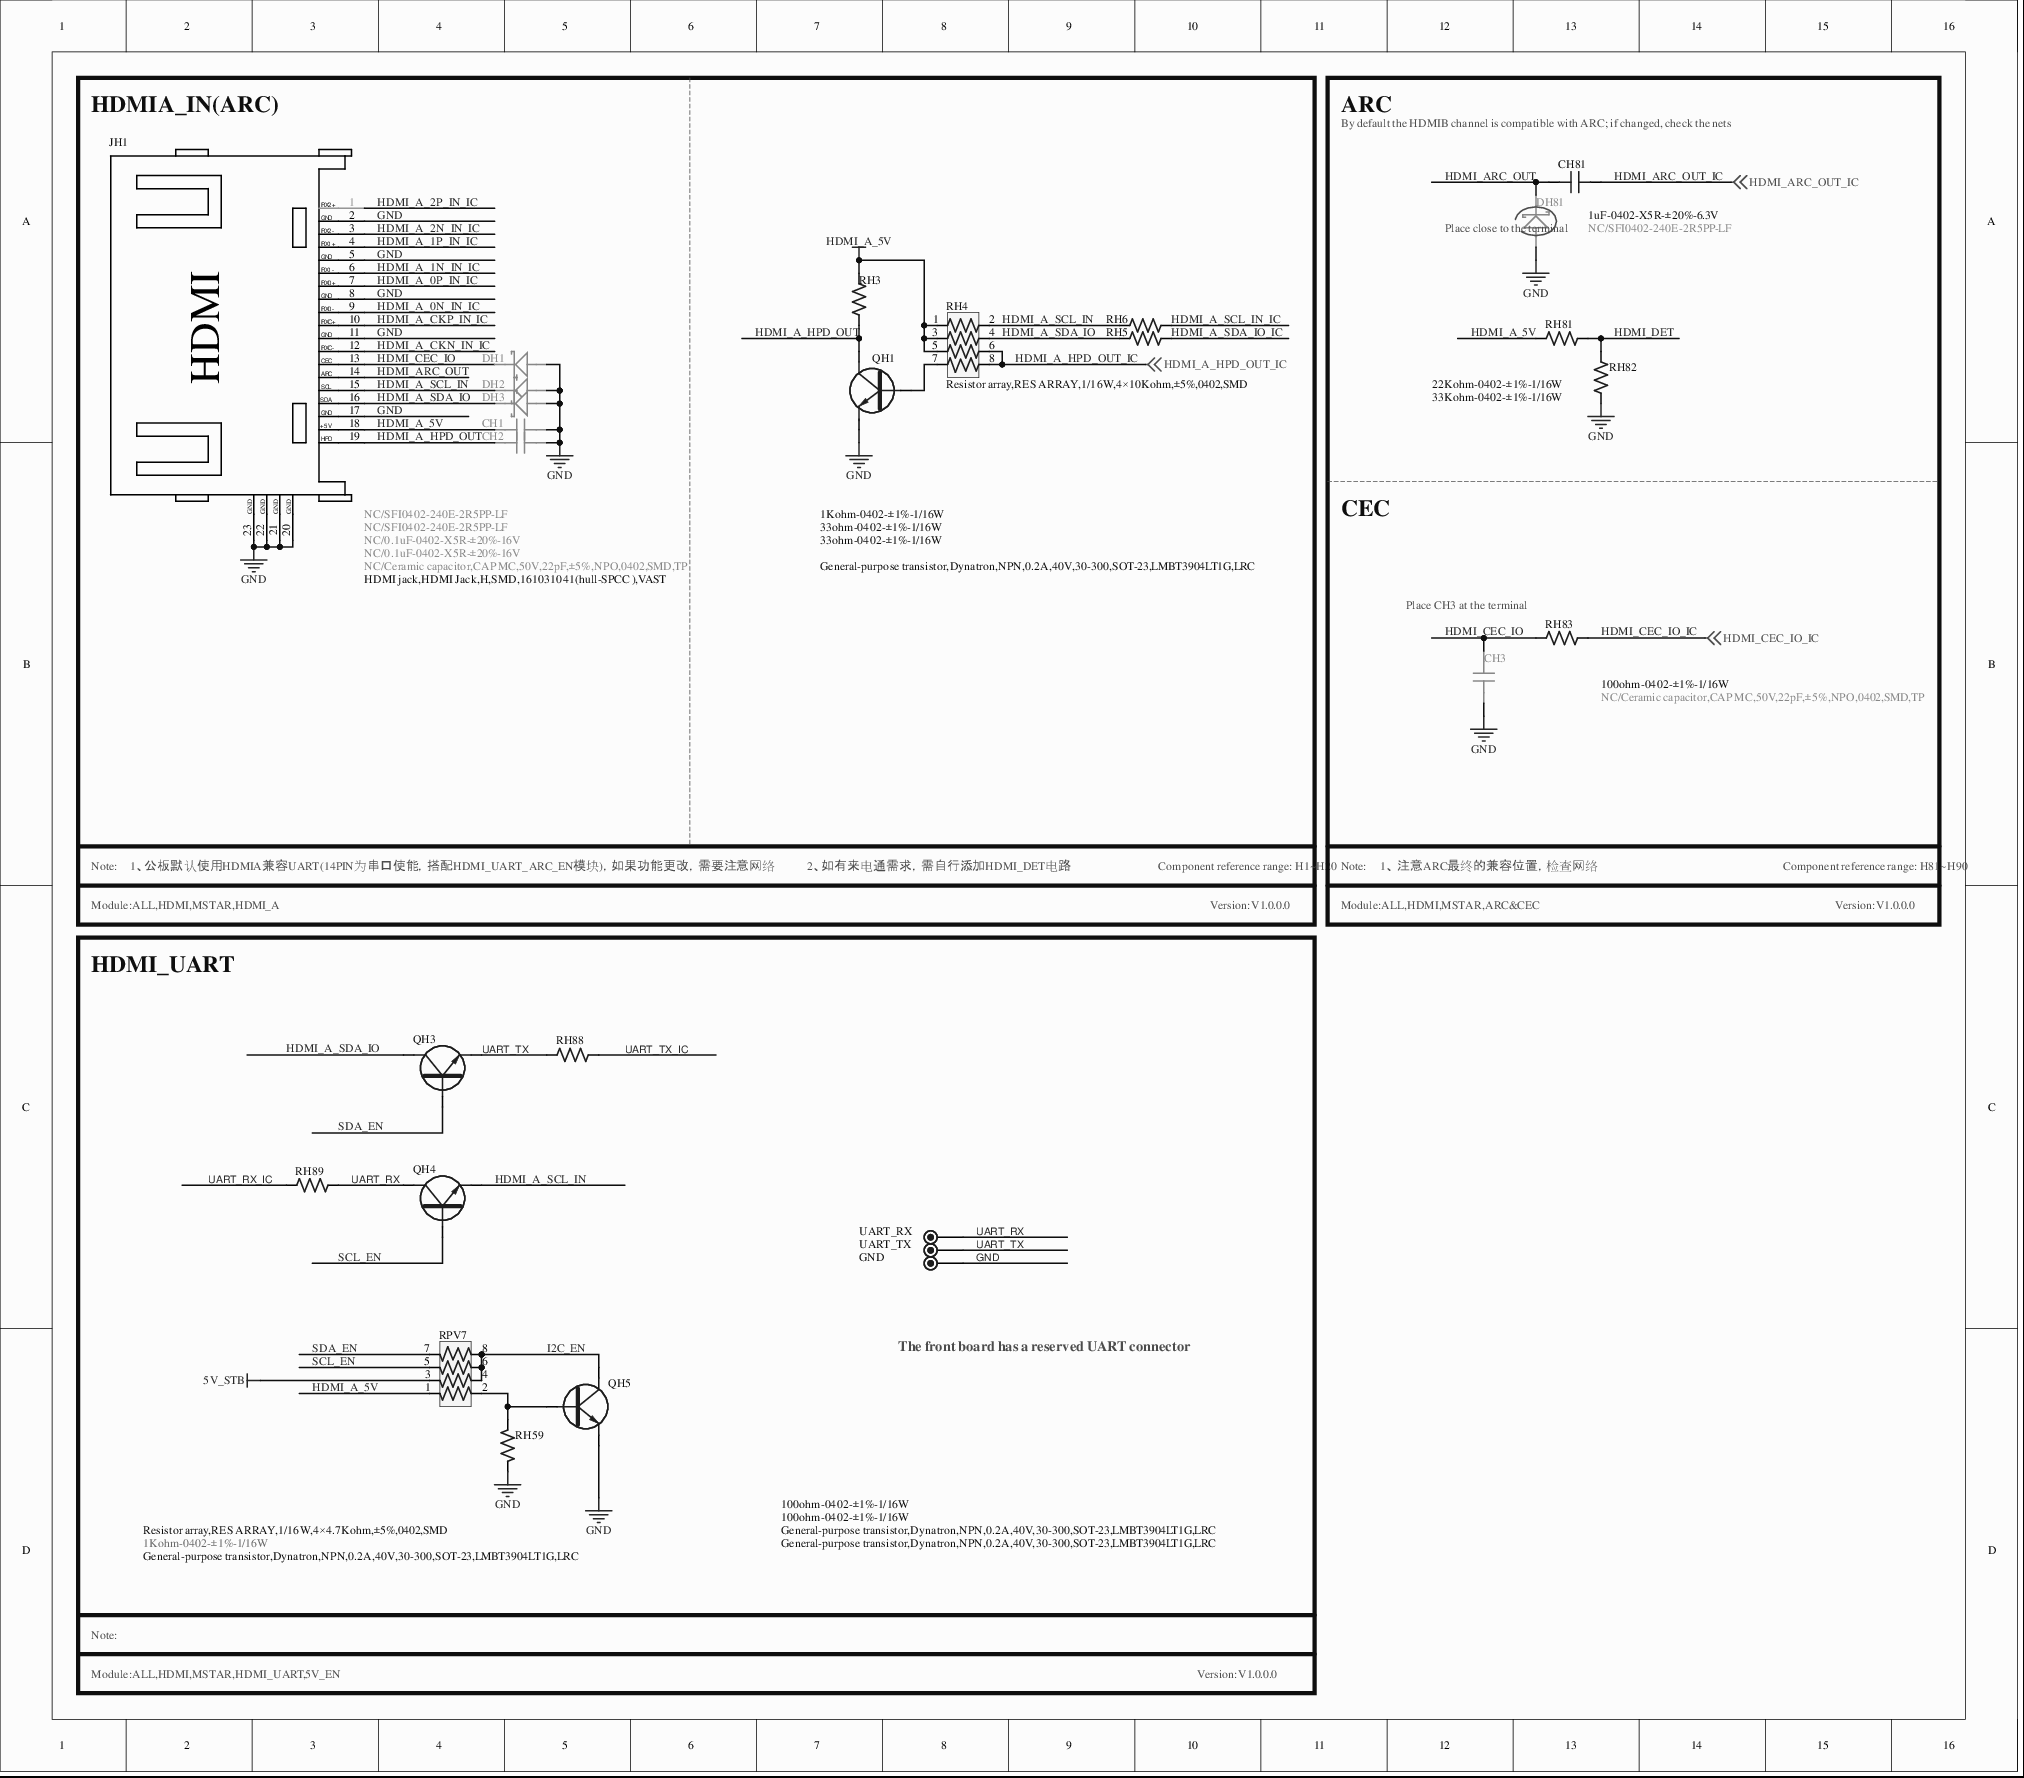
[diagram p0: MISC116569-11.SchDoc]
# Altium project MISC116569-15.PrjPCB (part 6 of 8)

## Sheet MISC116569-11.SchDoc
size 393 x 345 mm

### Parts
CH1  NC/0.1uF-0402-X5R-±20%-16V  [C0402]
CH2  NC/0.1uF-0402-X5R-±20%-16V  [C0402]
CH3  NC/Ceramic capacitor,CAP MC,50V,22pF,±5%,NPO,0402,SMD,TP  [C0402]
CH81  1uF-0402-X5R-±20%-6.3V  [C0402]
DH1  NC/Ceramic capacitor,CAP MC,50V,22pF,±5%,NPO,0402,SMD,TP  [DIODE-S0402]
DH2  NC/SFI0402-240E-2R5PP-LF  [DIODE-S0402]
DH3  NC/SFI0402-240E-2R5PP-LF  [DIODE-S0402]
DH81  NC/SFI0402-240E-2R5PP-LF  [DIODE-S0402]
GND  (no value)  [TP]
JH1  HDMI jack,HDMI Jack,H,SMD,161031041(hull-SPCC ),VAST  [HDMI-HS-1]
QH1  General-purpose transistor,Dynatron,NPN,0.2A,40V,30-300,SOT-23,LMBT3904LT1G,LRC  [SOT-23]
QH3  General-purpose transistor,Dynatron,NPN,0.2A,40V,30-300,SOT-23,LMBT3904LT1G,LRC  [SOT-23]
QH4  General-purpose transistor,Dynatron,NPN,0.2A,40V,30-300,SOT-23,LMBT3904LT1G,LRC  [SOT-23]
QH5  General-purpose transistor,Dynatron,NPN,0.2A,40V,30-300,SOT-23,LMBT3904LT1G,LRC  [SOT-23]
RH3  1Kohm-0402-±1%-1/16W  [R0402]
RH4  Resistor array,RES ARRAY,1/16W,4×10Kohm,±5%,0402,SMD  [RA0402]
RH5  33ohm-0402-±1%-1/16W  [R0402]
RH6  33ohm-0402-±1%-1/16W  [R0402]
RH59  1Kohm-0402-±1%-1/16W  [R0402]
RH81  22Kohm-0402-±1%-1/16W  [R0402]
RH82  33Kohm-0402-±1%-1/16W  [R0402]
RH83  100ohm-0402-±1%-1/16W  [R0402]
RH88  100ohm-0402-±1%-1/16W  [R0402]
RH89  100ohm-0402-±1%-1/16W  [R0402]
RPV7  Resistor array,RES ARRAY,1/16W,4×4.7Kohm,±5%,0402,SMD  [RA0402]
UART_RX  (no value)  [TP]
UART_TX  (no value)  [TP]

### Blocks framed on the sheet
HDMIA_IN(ARC): CH1 CH2 DH1-DH3 JH1 QH1 RH3-RH6
HDMI_UART: GND QH3-QH5 RH59 RH88 RH89 RPV7 UART_RX UART_TX

### Nets
5V_STB: RPV7.3
GND: CH1.2 CH2.2 CH3.1 DH1.A DH2.A DH3.A DH81.A GND.1 JH1.2 JH1.5 JH1.8 JH1.11 JH1.17 JH1.20 JH1.21 JH1.22 JH1.23 QH1.E QH5.E RH59.1 RH82.2
HDMI_A_5V: CH1.1 JH1.18 RH3.2 RH4.1 RH4.3 RH4.5 RH81.2 RPV7.1
HDMI_A_0N_IN_IC: JH1.9
HDMI_A_0P_IN_IC: JH1.7
HDMI_A_1N_IN_IC: JH1.6
HDMI_A_1P_IN_IC: JH1.4
HDMI_A_2N_IN_IC: JH1.3
HDMI_A_2P_IN_IC: JH1.1
HDMI_A_CKN_IN_IC: JH1.12
HDMI_A_CKP_IN_IC: JH1.10
HDMI_A_HPD_OUT: CH2.1 JH1.19 QH1.C RH3.1
HDMI_A_HPD_OUT_IC: RH4.6 RH4.8 ; off-sheet HDMI_A_HPD_OUT_IC
HDMI_A_SCL_IN: DH2.K JH1.15 QH4.E RH4.2 RH6.1
HDMI_A_SCL_IN_IC: RH6.2
HDMI_A_SDA_IO: DH3.K JH1.16 QH3.C RH4.4 RH5.1
HDMI_A_SDA_IO_IC: RH5.2
HDMI_ARC_OUT: CH81.1 DH81.K JH1.14
HDMI_ARC_OUT_IC: CH81.2 ; off-sheet HDMI_ARC_OUT_IC
HDMI_CEC_IO: CH3.2 DH1.K JH1.13 RH83.2
HDMI_CEC_IO_IC: RH83.1 ; off-sheet HDMI_CEC_IO_IC
HDMI_DET: RH81.1 RH82.1
I2C_EN: QH5.C RPV7.4 RPV7.6 RPV7.8
SCL_EN: QH4.B RPV7.5
SDA_EN: QH3.B RPV7.7
UART_RX: QH4.C RH89.1 UART_RX.1
UART_RX_IC: RH89.2
UART_TX: QH3.E RH88.2 UART_TX.1
UART_TX_IC: RH88.1
NetQH1_B: QH1.B RH4.7
NetQH5_B: QH5.B RH59.2 RPV7.2

### Notes on the sheet
- ARC
- By default the HDMIB channel is compatible with ARC; if changed, check the nets
- (near DH81) Place close to the terminal
- CEC
- (near RH83) Place CH3 at the terminal
- Note:
- 1、公板默认使用HDMIA兼容UART(14PIN为串口使能，搭配HDMI_UART_ARC_EN模块)，如果功能更改，需要注意网络
- 2、如有来电通需求，需自行添加HDMI_DET电路
- Component reference range: H1~H20
- 1、 注意ARC最终的兼容位置，检查网络
- Component reference range: H81~H90
- Module:ALL,HDMI,MSTAR,HDMI_A
- Version:V1.0.0.0
- Module:ALL,HDMI,MSTAR,ARC&CEC
- The front board has a reserved UART connector
- Module:ALL,HDMI,MSTAR,HDMI_UART,5V_EN

### Library data of the parts
CH1 CH2 = 0.1uF-0402-X5R-±20%-16V-D
CH3 = 004.003.0000530-D: Ceramic capacitor,CAP MC,50V,22pF,±5%,NPO,0402,SMD,TP-D
CH81 = 1uF-0402-X5R-±20%-6.3V-D
DH1-DH3 DH81 = 004.005.0000315-D: TVS diode,DIO ESD,2.5pF,200V,0402,SMD,SFI0402-240E-2R5PP-LF,SFI-D
GND UART_RX UART_TX = TEST
JH1 = XXX.XXX.0001122-D: HDMI jack,HDMI Jack,H,SMD,161031041(hull-SPCC ),VAST-D
QH1 = 004.006.0000007-D: General-purpose transistor,Dynatron,NPN,0.2A,40V,60-300,SOT-23,KMBT3904,KEXIN-D
QH3-QH5 = LMBT3904LT1G-D-NPN: Q-NPN-#-#-#
RH3 = 1Kohm-0402-±5%-1/16W-D
RH4 RPV7 = 4*100ohm-0402-±5%-1/16W-D
RH5 RH6 = 33ohm-0402-±5%-1/16W-D
RH59 = 10Kohm-0402-±5%-1/16W-D
RH81 = 22Kohm-0402-±5%-1/16W-D
RH82 = 33Kohm-0402-±5%-1/16W-D
RH83 RH88 RH89 = 004.002.0000568-D: Thick-film resistor,RES,1/16W,100ohm,±5%,0402,SMD-D

## Sheet MISC116569-12.SchDoc
size 294 x 215 mm
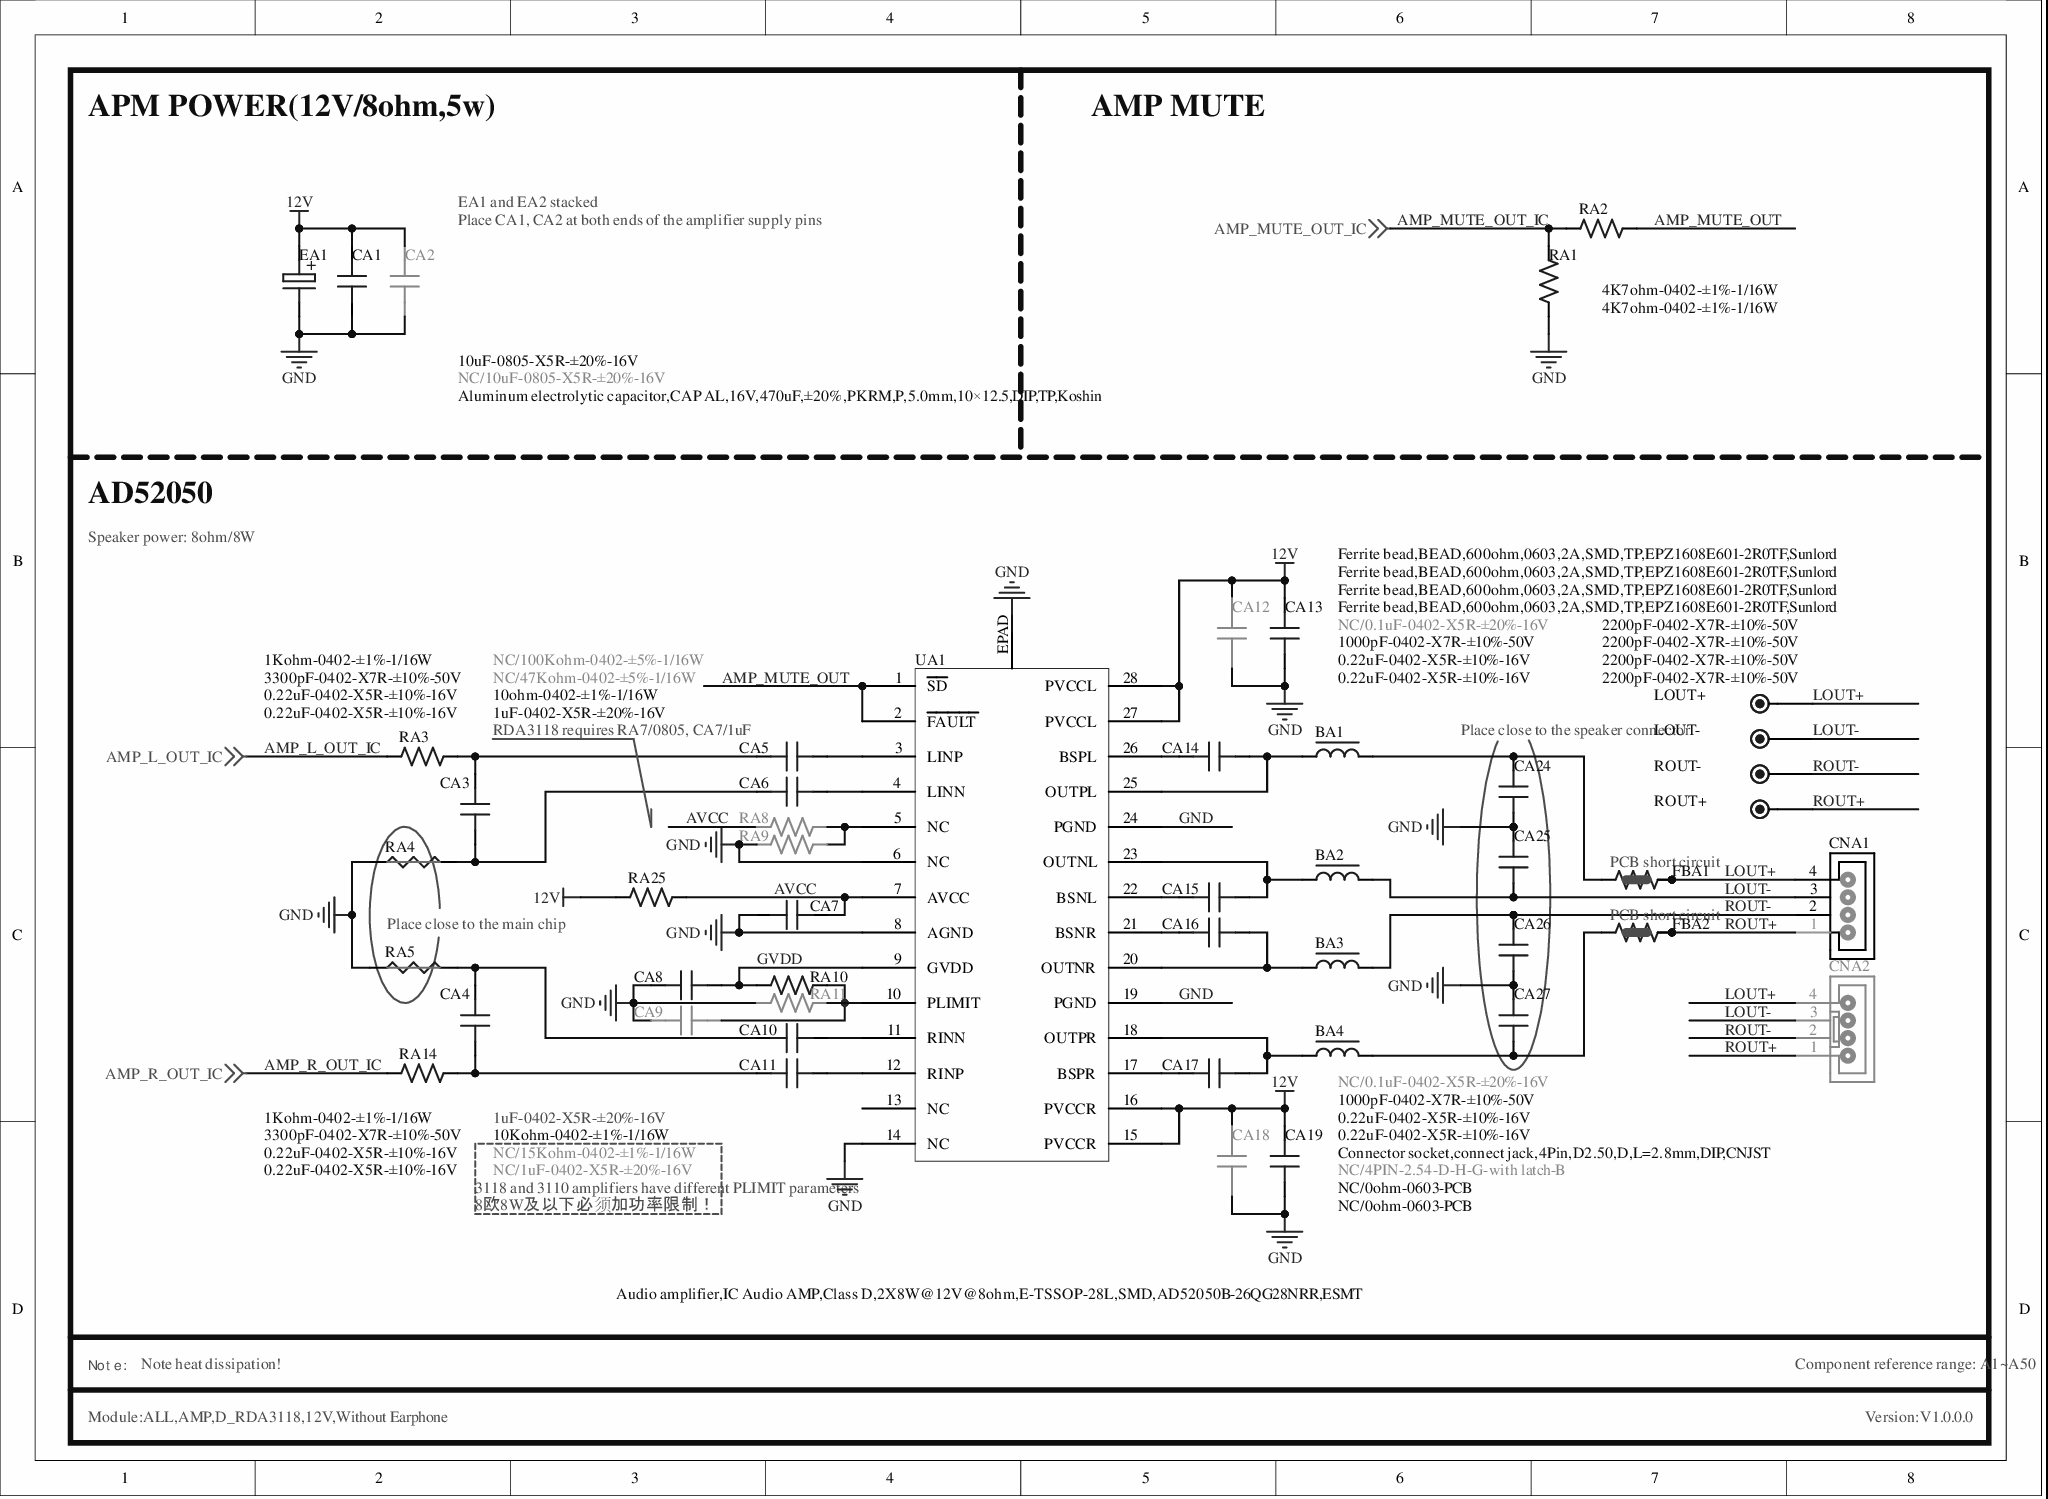
[diagram p1: MISC116569-12.SchDoc]

### Parts
BA1  Ferrite bead,BEAD,600ohm,0603,2A,SMD,TP,EPZ1608E601-2R0TF,Sunlord  [L0603]
BA2  Ferrite bead,BEAD,600ohm,0603,2A,SMD,TP,EPZ1608E601-2R0TF,Sunlord  [L0603]
BA3  Ferrite bead,BEAD,600ohm,0603,2A,SMD,TP,EPZ1608E601-2R0TF,Sunlord  [L0603]
BA4  Ferrite bead,BEAD,600ohm,0603,2A,SMD,TP,EPZ1608E601-2R0TF,Sunlord  [L0603]
CA1  10uF-0805-X5R-±20%-16V  [C0805]
CA2  NC/10uF-0805-X5R-±20%-16V  [C0805]
CA3  3300pF-0402-X7R-±10%-50V  [C0402]
CA4  3300pF-0402-X7R-±10%-50V  [C0402]
CA5  0.22uF-0402-X5R-±10%-16V  [C0402]
CA6  0.22uF-0402-X5R-±10%-16V  [C0402]
CA7  1uF-0402-X5R-±20%-16V  [C0402]
CA8  1uF-0402-X5R-±20%-16V  [C0402]
CA9  NC/1uF-0402-X5R-±20%-16V  [C0402]
CA10  0.22uF-0402-X5R-±10%-16V  [C0402]
CA11  0.22uF-0402-X5R-±10%-16V  [C0402]
CA12  NC/0.1uF-0402-X5R-±20%-16V  [C0402]
CA13  1000pF-0402-X7R-±10%-50V  [C0402]
CA14  0.22uF-0402-X5R-±10%-16V  [C0402]
CA15  0.22uF-0402-X5R-±10%-16V  [C0402]
CA16  0.22uF-0402-X5R-±10%-16V  [C0402]
CA17  0.22uF-0402-X5R-±10%-16V  [C0402]
CA18  NC/0.1uF-0402-X5R-±20%-16V  [C0402]
CA19  1000pF-0402-X7R-±10%-50V  [C0402]
CA24  2200pF-0402-X7R-±10%-50V  [C0402]
CA25  2200pF-0402-X7R-±10%-50V  [C0402]
CA26  2200pF-0402-X7R-±10%-50V  [C0402]
CA27  2200pF-0402-X7R-±10%-50V  [C0402]
CNA1  Connector socket,connect jack,4Pin,D2.50,D,L=2.8mm,DIP,CNJST  [SIP4/2.54D-1]
CNA2  NC/4PIN-2.54-D-H-G-with latch-B  [SIP4/2.5D-2]
EA1  Aluminum electrolytic capacitor,CAP AL,16V,470uF,±20%,PKRM,P,5.0mm,10×12.5,DIP,TP,Koshin  [EC(10*12)-V-5]
FBA1  NC/0ohm-0603-PCB  [R0603SC]
FBA2  NC/0ohm-0603-PCB  [R0603SC]
LOUT+  DM0  [TP]  (value not drawn)
LOUT-  DM0  [TP]  (value not drawn)
RA1  4K7ohm-0402-±1%-1/16W  [R0402]
RA2  4K7ohm-0402-±1%-1/16W  [R0402]
RA3  1Kohm-0402-±1%-1/16W  [R0402]
RA4  NC/?  [GND]  (value not drawn)
RA5  NC/?  [GND]  (value not drawn)
RA8  NC/100Kohm-0402-±5%-1/16W  [R0402]
RA9  NC/47Kohm-0402-±5%-1/16W  [R0402]
RA10  10Kohm-0402-±1%-1/16W  [R0402]
RA11  NC/15Kohm-0402-±1%-1/16W  [R0402]
RA14  1Kohm-0402-±1%-1/16W  [R0402]
RA25  10ohm-0402-±1%-1/16W  [R0402]
ROUT+  DM0  [TP]  (value not drawn)
ROUT-  DM0  [TP]  (value not drawn)
UA1  Audio amplifier,IC Audio AMP,Class D,2X8W@12V@8ohm,E-TSSOP-28L,SMD,AD52050B-26QG28NRR,ESMT  [SOP28/0.65-7]

### Nets
12V: CA1.2 CA2.2 CA12.2 CA13.2 CA18.2 CA19.2 EA1.1 RA25.2 UA1.15(PVCCR) UA1.16(PVCCR) UA1.27(PVCCL) UA1.28(PVCCL)
GND: CA1.1 CA2.1 CA7.1 CA8.1 CA9.1 CA12.1 CA13.1 CA18.1 CA19.1 CA24.1 CA25.2 CA26.1 CA27.2 EA1.2 RA1.2 RA4.JP_2K RA5.JP_2K RA9.1 RA11.1 UA1.6(NC) UA1.8(AGND) UA1.14(NC) UA1.19(PGND) UA1.24(PGND) UA1.EPAD
AMP_L_OUT_IC: RA3.1 ; off-sheet AMP_L_OUT_IC
AMP_MUTE_OUT: RA2.1 UA1.1(~{SD}) UA1.2(~{FAULT})
AMP_MUTE_OUT_IC: RA1.1 RA2.2 ; off-sheet AMP_MUTE_OUT_IC
AMP_R_OUT_IC: RA14.1 ; off-sheet AMP_R_OUT_IC
AVCC: CA7.2 RA8.1 RA25.1 UA1.7(AVCC)
GVDD: CA8.2 RA10.1 UA1.9(GVDD)
LOUT+: CNA1.4 CNA2.4 FBA1.2 FBA1.3 LOUT+.1
LOUT-: BA2.2 CA25.1 CNA1.3 CNA2.3 LOUT-.1
ROUT+: CNA1.1 CNA2.1 FBA2.2 FBA2.3 ROUT+.1
ROUT-: BA3.2 CA26.2 CNA1.2 CNA2.2 ROUT-.1
NetBA1_1: BA1.1 CA14.2 UA1.25(OUTPL)
NetBA1_2: BA1.2 CA24.2 FBA1.1
NetBA2_1: BA2.1 CA15.2 UA1.23(OUTNL)
NetBA3_1: BA3.1 CA16.2 UA1.20(OUTNR)
NetBA4_1: BA4.1 CA17.2 UA1.18(OUTPR)
NetBA4_2: BA4.2 CA27.1 FBA2.1
NetCA3_1: CA3.1 CA6.1 RA4.JP_1K
NetCA3_2: CA3.2 CA5.1 RA3.2
NetCA4_1: CA4.1 CA11.1 RA14.2
NetCA4_2: CA4.2 CA10.1 RA5.JP_1K
NetCA5_2: CA5.2 UA1.3(LINP)
NetCA6_2: CA6.2 UA1.4(LINN)
NetCA9_2: CA9.2 RA10.2 RA11.2 UA1.10(PLIMIT)
NetCA10_2: CA10.2 UA1.11(RINN)
NetCA11_2: CA11.2 UA1.12(RINP)
NetCA14_1: CA14.1 UA1.26(BSPL)
NetCA15_1: CA15.1 UA1.22(BSNL)
NetCA16_1: CA16.1 UA1.21(BSNR)
NetCA17_1: CA17.1 UA1.17(BSPR)
NetRA8_2: RA8.2 RA9.2 UA1.5(NC)

Not connected (* = marked no-connect by the designer): UA1 13(NC)*

### Notes on the sheet
- APM POWER(12V/8ohm,5w)
- AMP MUTE
- EA1 and EA2 stacked
- (near CA2) Place CA1, CA2 at both ends of the amplifier supply pins
- AD52050
- Speaker power: 8ohm/8W
- (near CA5) RDA3118 requires RA7/0805, CA7/1uF
- Place close to the speaker connector
- Place close to the main chip
- (near UA1) 3118 and 3110 amplifiers have different PLIMIT parameters
- 8欧8W及以下必须加功率限制！
- Note:
- Module:ALL,AMP,D_RDA3118,12V,Without Earphone
- Note heat dissipation!
- Component reference range: A1~A50
- Version:V1.0.0.0

### Library data of the parts
BA1-BA4 = 004.004.0000104-D: Multilayer inductor,HF Inductor,220nH,±5%,0603,SMD,SWI0603F-R22J,Tai-tech-D
CA1 CA2 = 004.003.0000386-D: Ceramic capacitor,CAP MC,16V,10uF,±20%,X5R,0805,SMD,TP-D
CA3 CA4 = 004.003.0000549-D: Ceramic capacitor,CAP MC,50V,3300pF,±10%,X7R,0402,SMD,TP-D
CA5 CA6 CA10 CA11 CA14-CA17 = 004.003.0000398-D: Ceramic capacitor,CAP MC,16V,0.22uF,±20%,X5R,0402,SMD,TP-D
CA7 CA9 = 004.003.0000402-D: Ceramic capacitor,CAP MC,16V,1uF,±20%,X5R,0402,SMD,TP-D
CA8 CA12 CA18 = 004.003.0000403-D: Ceramic capacitor,CAP MC,16V,0.1uF,±20%,X5R,0402,SMD,TP-D
CA13 CA19 = 004.003.0000503-D: Ceramic capacitor,CAP MC,50V,1000pF,±10%,X7R,0402,SMD,TP-D
CA24-CA27 = 004.003.0000534-D: Ceramic capacitor,CAP MC,50V,2200pF,±10%,X7R,0402,SMD,TP-D
CNA1 = XXX.XXX.0000595-DHMI: Connector socket,connect jack,4Pin,D2.50,D,L=2.8mm,DIP,CNJST-DHMI
CNA2 = XXX.XXX.0000676-DHMI: Connector socket,connect jack,4Pin,D2.54,D,SNAP,L=3.0mm,DIP,BOOM-DHMI
EA1 = 004.003.0000601-DHAI: Aluminum electrolytic capacitor,CAP AL,16V,470uF,±20%,RK,P,5.0mm,10×12,DIP,TP,XL-DHAI
FBA1 FBA2 = 0ohm-0603-PCB-D
LOUT+ LOUT- ROUT+ ROUT- = TEST
RA1 RA2 = 004.002.0000689-D: Thick-film resistor,RES,1/16W,4.7Kohm,±5%,0402,SMD-D
RA3 RA14 = 004.002.0000572-D: Thick-film resistor,RES,1/16W,1Kohm,±5%,0402,SMD-D
RA4 RA5 = GND: Manufacturer: Panasonic; Part Number: ERJ3GEYJ473V; Right: 20; Bottom: 30; CLASS: Discrete; Comments: Digikey
RA8 = 004.002.0000579-D: Thick-film resistor,RES,1/16W,100Kohm,±5%,0402,SMD-D
RA9 = 004.002.0000691-D: Thick-film resistor,RES,1/16W,47Kohm,±5%,0402,SMD-D
RA10 = 004.002.0000575-D: Thick-film resistor,RES,1/16W,10Kohm,±1%,0402,SMD-D
RA11 = 004.002.0000602-D: Thick-film resistor,RES,1/16W,15Kohm,±1%,0402,SMD-D
RA25 = 004.002.0000568-D: as RH83 on sheet MISC116569-11
UA1 = 004.012.0000275-D: Audio amplifier,IC Audio AMP,Class D,2X8W@12V@8ohm,E-TSSOP-28L,SMD,AD52050B-26QG28NRR,ESMT-D

## Sheet MISC116569-13.SchDoc
size 426 x 299 mm
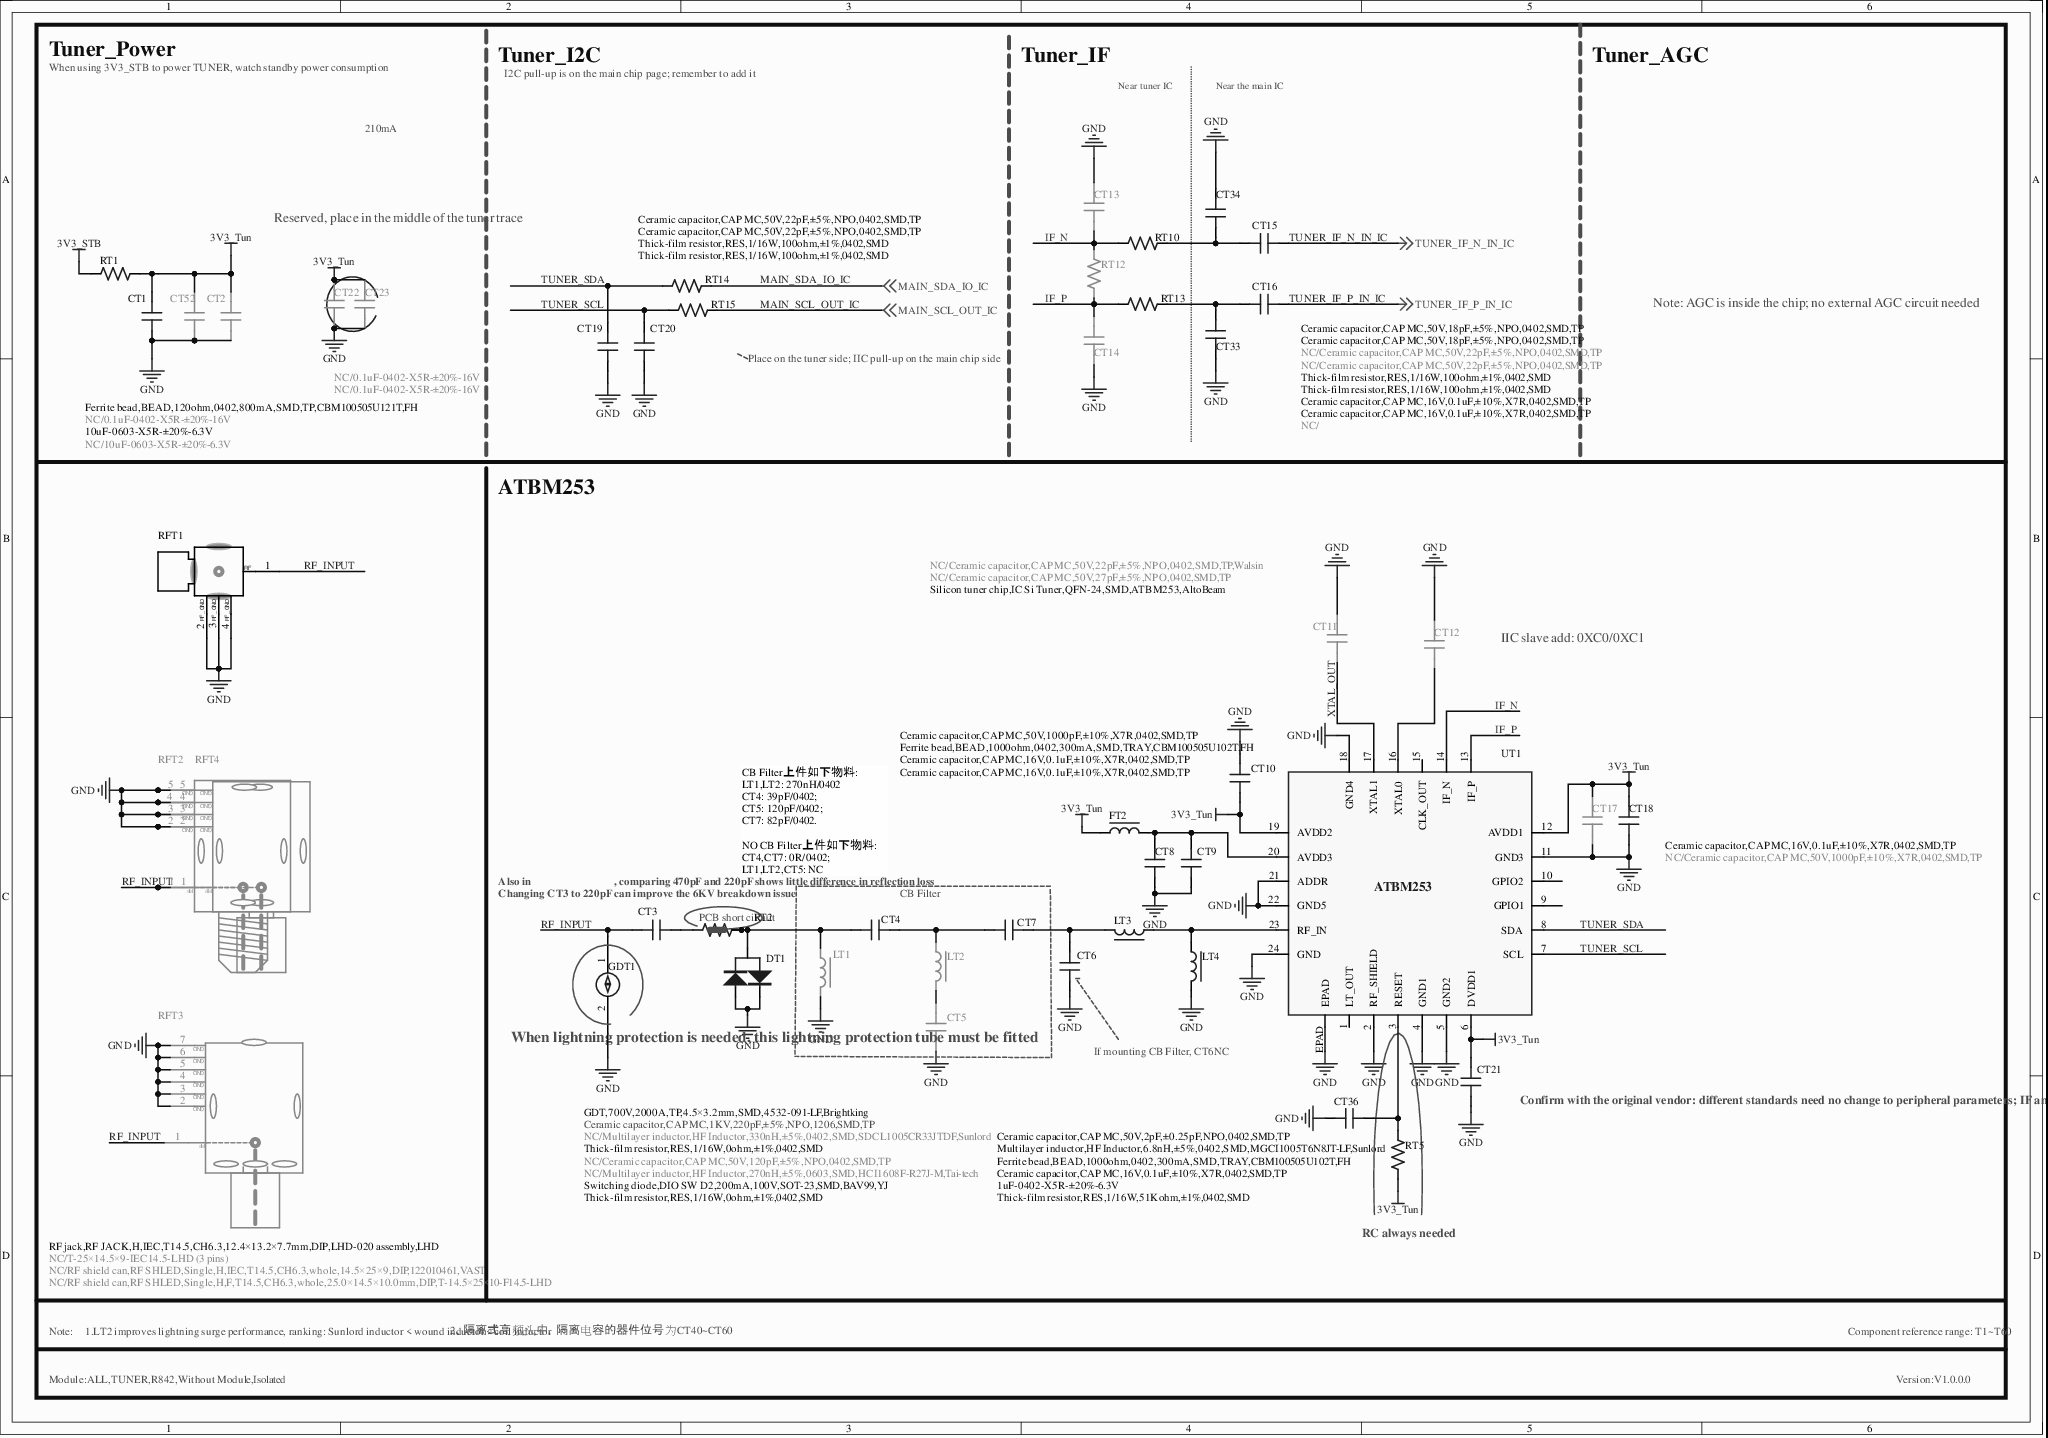
[diagram p2: MISC116569-13.SchDoc]

### Parts
CT1  10uF-0603-X5R-±20%-6.3V  [C0603]
CT2  NC/0.1uF-0402-X5R-±20%-16V  [C0402]
CT3  Ceramic capacitor,CAP MC,1KV,220pF,±5%,NPO,1206,SMD,TP  [C1206]
CT4  Thick-film resistor,RES,1/16W,0ohm,±1%,0402,SMD  [C0402]
CT5  NC/Ceramic capacitor,CAP MC,50V,120pF,±5%,NPO,0402,SMD,TP  [C0402]
CT6  Ceramic capacitor,CAP MC,50V,2pF,±0.25pF,NPO,0402,SMD,TP  [C0402]
CT7  Thick-film resistor,RES,1/16W,0ohm,±1%,0402,SMD  [C0402]
CT8  Ceramic capacitor,CAP MC,16V,0.1uF,±10%,X7R,0402,SMD,TP  [C0402]
CT9  Ceramic capacitor,CAP MC,50V,1000pF,±10%,X7R,0402,SMD,TP  [C0402]
CT10  Ceramic capacitor,CAP MC,16V,0.1uF,±10%,X7R,0402,SMD,TP  [C0402]
CT11  NC/Ceramic capacitor,CAP MC,50V,22pF,±5%,NPO,0402,SMD,TP,Walsin  [C0402]
CT12  NC/Ceramic capacitor,CAP MC,50V,27pF,±5%,NPO,0402,SMD,TP  [C0402]
CT13  NC/Ceramic capacitor,CAP MC,50V,22pF,±5%,NPO,0402,SMD,TP  [C0402]
CT14  NC/Ceramic capacitor,CAP MC,50V,22pF,±5%,NPO,0402,SMD,TP  [C0402]
CT15  Ceramic capacitor,CAP MC,16V,0.1uF,±10%,X7R,0402,SMD,TP  [C0402]
CT16  Ceramic capacitor,CAP MC,16V,0.1uF,±10%,X7R,0402,SMD,TP  [C0402]
CT17  NC/Ceramic capacitor,CAP MC,50V,1000pF,±10%,X7R,0402,SMD,TP  [C0402]
CT18  Ceramic capacitor,CAP MC,16V,0.1uF,±10%,X7R,0402,SMD,TP  [C0402]
CT19  Ceramic capacitor,CAP MC,50V,22pF,±5%,NPO,0402,SMD,TP  [C0402]
CT20  Ceramic capacitor,CAP MC,50V,22pF,±5%,NPO,0402,SMD,TP  [C0402]
CT21  Ceramic capacitor,CAP MC,16V,0.1uF,±10%,X7R,0402,SMD,TP  [C0402]
CT22  NC/0.1uF-0402-X5R-±20%-16V  [C0402]
CT23  NC/0.1uF-0402-X5R-±20%-16V  [C0402]
CT33  Ceramic capacitor,CAP MC,50V,18pF,±5%,NPO,0402,SMD,TP  [C0402]
CT34  Ceramic capacitor,CAP MC,50V,18pF,±5%,NPO,0402,SMD,TP  [C0402]
CT36  1uF-0402-X5R-±20%-6.3V  [C0402]
CT52  NC/10uF-0603-X5R-±20%-6.3V  [C0603]
DT1  Switching diode,DIO SW D2,200mA,100V,SOT-23,SMD,BAV99,YJ  [SO-23]
FT2  Ferrite bead,BEAD,1000ohm,0402,300mA,SMD,TRAY,CBM100505U102T,FH  [L0402]
GDT1  GDT,700V,2000A,TP,4.5×3.2mm,SMD,4532-091-LF,Brightking  [SMD4532-1]
LT1  NC/Multilayer inductor,HF Inductor,330nH,±5%,0402,SMD,SDCL1005CR33JTDF,Sunlord  [L0402]
LT2  NC/Multilayer inductor,HF Inductor,270nH,±5%,0603,SMD,HCI1608F-R27J-M,Tai-tech  [L0603]
LT3  Multilayer inductor,HF Inductor,6.8nH,±5%,0402,SMD,MGCI1005T6N8JT-LF,Sunlord  [L0402]
LT4  Ferrite bead,BEAD,1000ohm,0402,300mA,SMD,TRAY,CBM100505U102T,FH  [L0402]
RFT1  RF jack,RF JACK,H,IEC,T14.5,CH6.3,12.4×13.2×7.7mm,DIP,LHD-020 assembly,LHD  [ANT-IEC14.5-H-4]
RFT2  NC/RF shield can,RF SHLED,Single,H,IEC,T14.5,CH6.3,whole,14.5×25×9,DIP,122010461,VAST  [T-14.5×25×9.0-IEC14.5]
RFT3  NC/T-25×14.5×9-IEC14.5-LHD (3 pins)  [T-25×14.5×9-IEC14.5-LHD-1]
RFT4  NC/RF shield can,RF SHLED,Single,H,F,T14.5,CH6.3,whole,25.0×14.5×10.0mm,DIP,T-14.5×25×10-F14.5-LHD  [T-14.5×25×10-F14.5]
RT1  Ferrite bead,BEAD,120ohm,0402,800mA,SMD,TP,CBM100505U121T,FH  [R0402]
RT2  NC/  [R0402SC]  (value not drawn)
RT5  Thick-film resistor,RES,1/16W,51Kohm,±1%,0402,SMD  [R0402]
RT10  Thick-film resistor,RES,1/16W,100ohm,±1%,0402,SMD  [R0402]
RT12  NC/  [R0402]
RT13  Thick-film resistor,RES,1/16W,100ohm,±1%,0402,SMD  [R0402]
RT14  Thick-film resistor,RES,1/16W,100ohm,±1%,0402,SMD  [R0402]
RT15  Thick-film resistor,RES,1/16W,100ohm,±1%,0402,SMD  [R0402]
UT1  Silicon tuner chip,IC Si Tuner,QFN-24,SMD,ATBM253,AltoBeam  [QFN24/0.4-1]

### Blocks framed on the sheet
CB Filter: CT4 CT5 CT7 LT1 LT2

### Nets
3V3_STB: RT1.1
3V3_Tun: CT1.2 CT2.2 CT10.2 CT17.1 CT18.2 CT21.2 CT22.1 CT23.1 CT52.2 FT2.2 RT1.2 RT5.1 UT1.6(DVDD1) UT1.12(AVDD1) UT1.19(AVDD2)
GND: CT1.1 CT2.1 CT5.2 CT6.2 CT8.2 CT9.1 CT10.1 CT11.1 CT12.1 CT13.2 CT14.1 CT17.2 CT18.1 CT19.1 CT20.1 CT21.1 CT22.2 CT23.2 CT33.1 CT34.2 CT36.2 CT52.1 DT1.1 DT1.3 GDT1.2 LT1.1 LT4.1 RFT1.2 RFT1.3 RFT1.4 RFT2.2 RFT2.3 RFT2.4 RFT2.5 RFT3.2 RFT3.3 RFT3.4 RFT3.5 RFT3.6 RFT3.7 RFT4.2 RFT4.3 RFT4.4 RFT4.5 UT1.2(RF_SHIELD) UT1.4(GND1) UT1.5(GND2) UT1.11(GND3) UT1.18(GND4) UT1.21(ADDR) UT1.22(GND5) UT1.24(GND) UT1.EPAD
IF_N: CT13.1 RT10.1 RT12.2 UT1.14(IF_N)
IF_P: CT14.2 RT12.1 RT13.1 UT1.13(IF_P)
MAIN_SCL_OUT_IC: RT15.2 ; off-sheet MAIN_SCL_OUT_IC
MAIN_SDA_IO_IC: RT14.2 ; off-sheet MAIN_SDA_IO_IC
RF_INPUT: CT3.2 GDT1.1 RFT1.1 RFT2.1 RFT3.1 RFT4.1
TUNER_IF_N_IN_IC: CT15.2 ; off-sheet TUNER_IF_N_IN_IC
TUNER_IF_P_IN_IC: CT16.1 ; off-sheet TUNER_IF_P_IN_IC
TUNER_SCL: CT20.2 RT15.1 UT1.7(SCL)
TUNER_SDA: CT19.2 RT14.1 UT1.8(SDA)
XTAL_OUT: CT11.2 UT1.17(XTAL1)
NetCT3_1: CT3.1 RT2.1
NetCT4_1: CT4.1 CT7.2 LT2.1
NetCT4_2: CT4.2 DT1.2 LT1.2 RT2.2 RT2.3
NetCT5_1: CT5.1 LT2.2
NetCT6_1: CT6.1 CT7.1 LT3.1
NetCT8_1: CT8.1 CT9.2 FT2.1 UT1.20(AVDD3)
NetCT12_2: CT12.2 UT1.16(XTAL0)
NetCT15_1: CT15.1 CT34.1 RT10.2
NetCT16_2: CT16.2 CT33.2 RT13.2
NetCT36_1: CT36.1 RT5.2 UT1.3(RESET)
NetLT3_2: LT3.2 LT4.2 UT1.23(RF_IN)

Not connected (* = marked no-connect by the designer): UT1 1(LT_OUT)* 9(GPIO1)* 10(GPIO2)* 15(CLK_OUT)*

### Notes on the sheet
- Tuner_Power
- When using 3V3_STB to power TUNER, watch standby power consumption
- Tuner_I2C
- I2C pull-up is on the main chip page; remember to add it
- Tuner_IF
- Near tuner IC
- Near the main IC
- Tuner_AGC
- 210mA
- Reserved, place in the middle of the tuner trace
- (near CT14) Place on the tuner side; IIC pull-up on the main chip side
- Note: AGC is inside the chip; no external AGC circuit needed
- ATBM253
- IIC slave add: 0XC0/0XC1
- Changing CT3 to 220pF can improve the 6KV breakdown issue
- Also in XXXXXXXXXXXXXX, comparing 470pF and 220pF shows little difference in reflection loss
- CB Filter上件如下物料:
  LT1,LT2: 270nH/0402
  CT4: 39pF/0402;
  CT5: 120pF/0402;
  CT7: 82pF/0402.
  NO CB Filter上件如下物料:
  CT4,CT7: 0R/0402;
  LT1,LT2,CT5: NC
- (near CT5) When lightning protection is needed, this lightning protection tube must be fitted
- If mounting CB Filter, CT6NC
- Confirm with the original vendor: different standards need no change to peripheral parameters; IF amplitude is changed by software.
- RC always needed
- Note:
- 1.LT2 improves lightning surge performance, ranking: Sunlord inductor < wound inductor < coil inductor
- 2、隔离式高频头中，隔离电容的器件位号为CT40~CT60
- Component reference range: T1~T60
- Module:ALL,TUNER,R842,Without Module,Isolated
- Version:V1.0.0.0

### Library data of the parts
CT1 CT52 = 10uF-0603-X5R-±20%-6.3V-D
CT2 CT4-CT12 CT15-CT18 CT21-CT23 = 0.1uF-0402-Y5V-+80%-20%-16V-D
CT3 = 1000pF-1206-X7R-±20%-2000V-D
CT13 CT14 CT19 CT20 CT33 CT34 CT36 = 33pF-0402-NPO-±5%-50V-D
DT1 = BAV99-BR-D
FT2 LT1 LT3 LT4 = SDCL1005CR27JTDF(顺络)-D
GDT1 = 004.005.0000675: Gas discharge tube,GDT,700V,2000A,TP,4.5*3.2mm,SMD,4532-091-LF,Brightking-D
LT2 = MGLB1608M121T2R0-LF(120ohm-2000mA)-D
RFT1 = RF头,RF JACK,H,IEC,T14.5,CH6.3,12.4×13.2×7.7mm,DIP,LHD-020组件,LHD-DLMI: T-IEC-6.3mm-#-#
RFT2 = RF屏蔽罩,RF SHLED,Single,H,IEC,T14.5,CH6.3,whole,14.5×25×9,DIP,122010461,VAST-DLMI: T-IEC-14.5×25×9, head length 14.5-#-#
RFT3 = T-25×14.5×9-IEC14.5-LHD(3只脚)-DLMI: T-IEC-14.5×25×9, head length 14.5-one-piece 3 pins-#
RFT4 = RF屏蔽罩,RF SHLED,Single,H,F,T14.5,CH6.3,whole,25.0×14.5×10.0mm,DIP,T-14.5×25×10-F14.5-LHD (一体),LHD-DLMI: T-F-14.5×25×10, head length 14.5-#-#
RT1 = 0ohm-0402-±5%-1/16W-D
RT2 = 0ohm-0402-PCB-D
RT5 RT10 RT12-RT15 = 220ohm-0402-±5%-1/16W-D
UT1 = 004.014.0000255-D: Silicon tuner chip,IC Si Tuner,QFN-24,SMD,ATBM253,AltoBeam-D